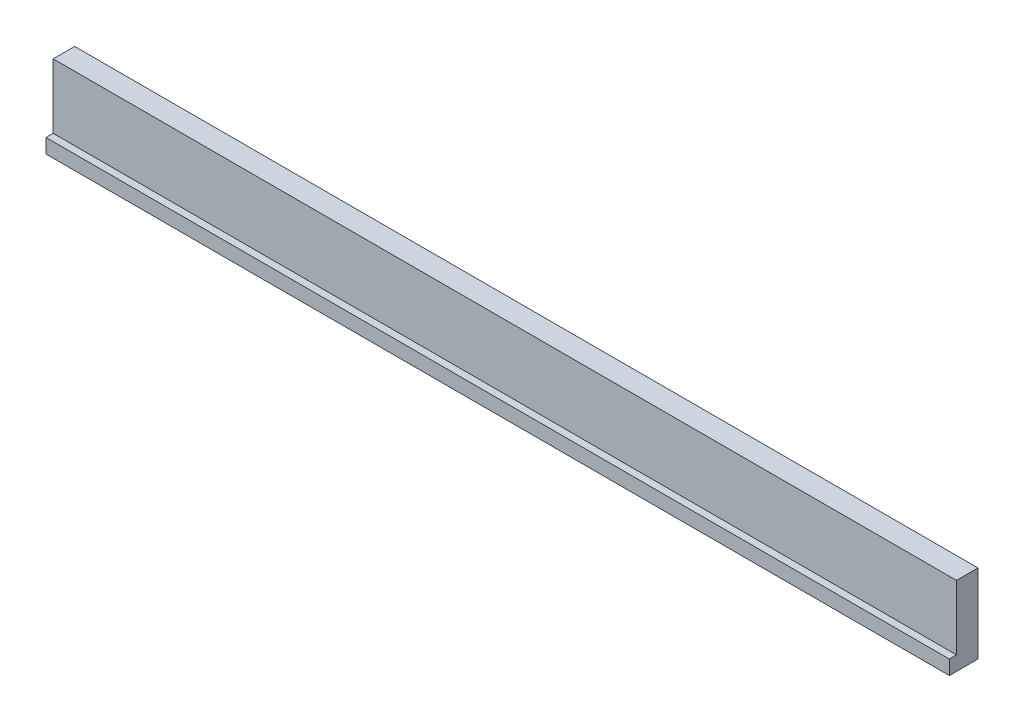
from build123d import *

# Parameters (mm, degrees)
BOSS_EXTRUDE1_DEPTH = 630


with BuildPart() as part:
    # Sketch1 → Boss-Extrude1 (new body)
    with BuildSketch(Plane(origin=(0, 0, 0), x_dir=(0, 0, -1), z_dir=(1, 0, 0))):
        Polygon((-31.215474357, 48.108563949), (-31.215474357, -6.891436051), (-51.215474357, -6.891436051), (-51.215474357, 3.108563949), (-46.215474357, 3.108563949), (-46.215474357, 48.108563949), align=None)
    extrude(amount=-BOSS_EXTRUDE1_DEPTH)


solid = part.part
